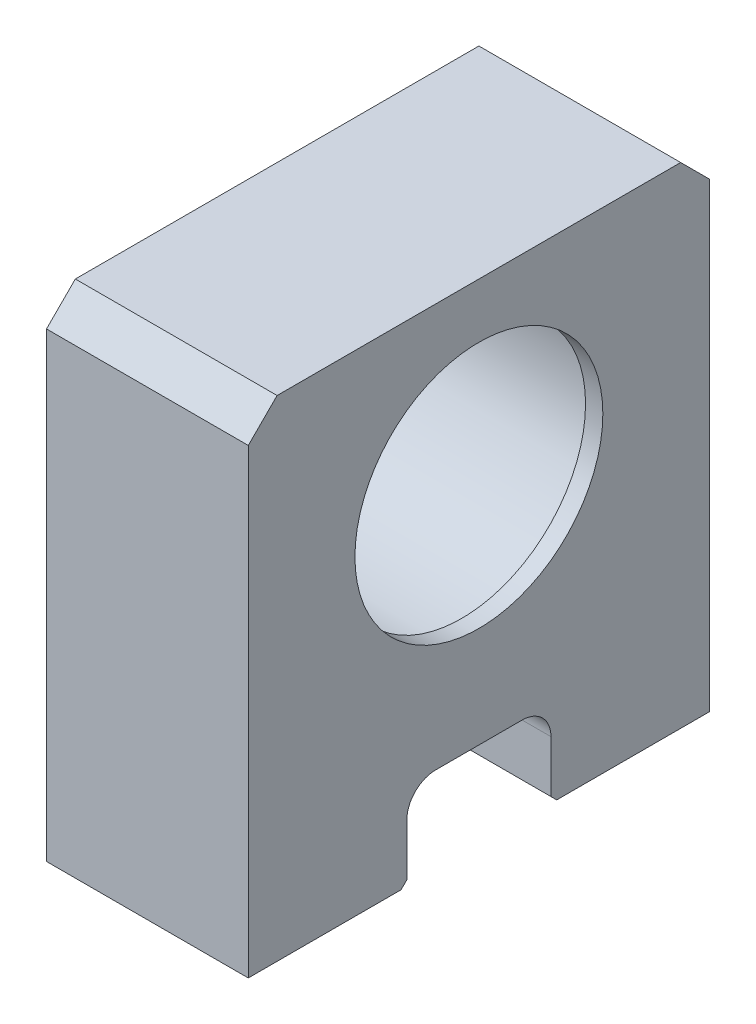
SolidWorks part; units mm, degrees
material "S45C"
ref_plane "Front Plane" through (0, 0, 0) normal (0, 0, 1) x (1, 0, 0)
ref_plane "Top Plane" through (0, 0, 0) normal (0, 1, 0) x (1, 0, 0)
ref_plane "Right Plane" through (0, 0, 0) normal (1, 0, 0) x (0, 0, -1)
sketch "Sketch1" plane through (0, 0, 0) normal (1, 0, 0) x (0, 0, -1)
  line L0 (-40, 85) -> (40, 85)
  line L1 (-40, 0) -> (-12.5, 0)
  line L2 (-40, 0) -> (-40, 85)
  line L3 (0, 0) -> (0, 44.2081) construction
  line L4 (40, 0) -> (40, 85)
  line L6 (-12.5, 0) -> (-12.5, 15)
  line L7 (-12.5, 15) -> (12.5, 15)
  line L8 (12.5, 0) -> (12.5, 15)
  line L9 (12.5, 0) -> (40, 0)
  circle A0 centre (0, 54) radius 21.5
  dimension "D3" = 43
  dimension "D4" = 54
  dimension "D1" = 85
  dimension "D2" = 80
  dimension "D5" = 25
  dimension "D6" = 15
extrude "Boss-Extrude1" add sketch "Sketch1" along normal mid plane 35
chamfer "Chamfer3" distance 5 angle 45 2 edges at (0, 85, -40) (0, 85, 40)
fillet "Fillet1" radius 5 2 edges at (0, 15, -12.5) (0, 15, 12.5)
hole_wizard "M6 Tapped Hole1" positions "Sketch9" profile "Sketch8" tap size "M6" standard "Gb"
sketch "Sketch9" plane through (0, 0, 0) normal (0, -1, 0) x (-1, 0, 0)
  line L0 (53.7796, 0) -> (-55.8319, 0) construction
  point P0 (0, -32.5)
  point P2 (0, 32.5)
  dimension "D1" = 65
sketch "Sketch8" plane through (0, 0, 32.5) normal (1, 0, 0) x (0, 0, -1)
  line L0 (0, 0) -> (0, 18.5022)
  line L1 (0, 18.5022) -> (2.5, 17)
  line L2 (2.5, 17) -> (2.5, 0)
  line L5 (2.5, 0) -> (0, 0)
  line L10 (0, 18.5022) -> (-2.5, 17) construction
  line L11 (0, -6.35) -> (0, 107.95) construction
  dimension "螺纹孔钻头直径" = 5
  dimension "螺纹孔钻头深度" = 17
  dimension "导头角度" = 118
cosmetic thread "Cosmetic Thread1" parameters "D1"=12, "D2"=6
cosmetic thread "Cosmetic Thread2" parameters "D1"=12, "D2"=6
sketch "Sketch11" plane through (0, 0, 0) normal (0, -1, 0) x (1, 0, 0)
  line L0 (32.5394, 0) -> (-27.4579, 0) construction
  line L1 (0, 40) -> (0, -40) construction
  line L2 (17.5, 40) -> (-17.5, 40) construction
  line L3 (17.5, -40) -> (-17.5, -40) construction
  line L4 (0, 20.5) -> (0, 19.5) construction
  line L5 (2.5, 20.5) -> (2.5, 19.5)
  line L6 (-2.5, 20.5) -> (-2.5, 19.5)
  arc A0 (2.5, 20.5) -> (-2.5, 20.5) centre (0, 20.5) ccw
  circle A1 centre (0, -20) radius 2.5
  arc A2 (-2.5, 19.5) -> (2.5, 19.5) centre (0, 19.5) ccw
  point P13 (0, 20)
  dimension "D1" = 5
  dimension "D2" = 40
  dimension "D3" = 1
extrude "Cut-Extrude1" cut sketch "Sketch11" against normal blind 15
chamfer "Chamfer4" distance 1 angle 45 2 edges at (0, 0, -12.5) (0, 0, 12.5)
sketch "Sketch12" plane through (-17.5, 0, 0) normal (-1, 0, 0) x (0, 0, 1)
  circle A0 centre (0, 54) radius 26
  dimension "D1" = 52
extrude "Cut-Extrude2" cut sketch "Sketch12" against normal blind 32
hole_wizard "M4 Tapped Hole1" positions "Sketch15" profile "Sketch14" tap size "M4" standard "Gb"
sketch "Sketch15" plane through (-17.5, 0, 0) normal (-1, 0, 0) x (0, 0, 1)
  line L0 (0, 54) -> (49.5275, 54) construction
  line L3 (0, 54) -> (0, 88.0615) construction
  point P0 (-22.5, 74)
  point P2 (22.5, 74)
  point P4 (22.5, 34)
  point P6 (-22.5, 34)
  dimension "D1" = 45
  dimension "D2" = 40
sketch "Sketch14" plane through (-17.5, 74, -22.5) normal (0, 1, 0) x (0, 0, 1)
  line L0 (0, 0) -> (0, 12.4914)
  line L1 (0, 12.4914) -> (1.65, 11.5)
  line L2 (1.65, 11.5) -> (1.65, 0)
  line L5 (1.65, 0) -> (0, 0)
  line L10 (0, 12.4914) -> (-1.65, 11.5) construction
  line L11 (0, -6.35) -> (0, 107.95) construction
  dimension "螺纹孔钻头直径" = 3.3
  dimension "螺纹孔钻头深度" = 11.5
  dimension "导头角度" = 118
cosmetic thread "Cosmetic Thread6" parameters "D1"=8, "D2"=4
cosmetic thread "Cosmetic Thread7" parameters "D1"=8, "D2"=4
cosmetic thread "Cosmetic Thread8" parameters "D1"=8, "D2"=4
cosmetic thread "Cosmetic Thread9" parameters "D1"=8, "D2"=4
chamfer "Chamfer5" distance 0.5 angle 45 1 edges at (-17.5, 54, 26)
